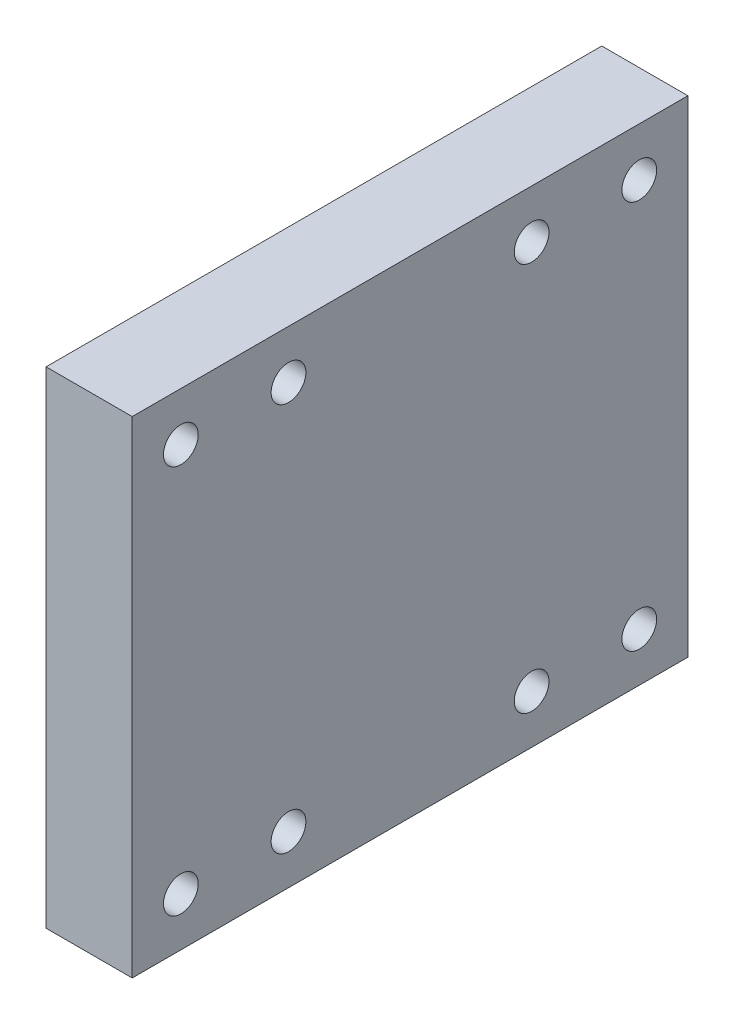
SolidWorks part; units mm, degrees
ref_plane "前视基准面" through (0, 0, 0) normal (0, 0, 1) x (1, 0, 0)
ref_plane "上视基准面" through (0, 0, 0) normal (0, 1, 0) x (1, 0, 0)
ref_plane "右视基准面" through (0, 0, 0) normal (1, 0, 0) x (0, 0, -1)
sketch "草图1" plane through (0, 0, 0) normal (1, 0, 0) x (0, 0, -1)
  line L1 (-40, 35) -> (40, 35)
  line L2 (-40, 35) -> (-40, -35)
  line L3 (-40, -35) -> (40, -35)
  line L4 (40, 35) -> (40, -35)
  line L5 (-40, 35) -> (40, -35) construction
  line L6 (-40, -35) -> (40, 35) construction
  point P0 (0, 0)
  dimension "D1" = 80
  dimension "D2" = 70
extrude "凸台-拉伸1" add sketch "草图1" along normal blind 12.4
hole_wizard "M6 螺纹孔1" positions "草图2" profile "草图3" tap size "M6" standard "GB"
sketch "草图2" plane through (12.4, 0, 0) normal (1, 0, 0) x (0, 0, -1)
  line L0 (0, 40.8734) -> (0, 0) construction
  line L1 (0, 0) -> (49.0326, 0) construction
  point P0 (-17.5, 28)
  point P2 (17.5, 28)
  point P4 (-17.5, -28)
  point P6 (17.5, -28)
  dimension "D1" = 35
  dimension "D2" = 56
sketch "草图3" plane through (12.4, 28, 17.5) normal (0, 1, 0) x (0, 0, -1)
  line L0 (0, 0) -> (0, 16.5022)
  line L1 (0, 16.5022) -> (2.5, 15)
  line L2 (2.5, 15) -> (2.5, 0)
  line L5 (2.5, 0) -> (0, 0)
  line L10 (0, 16.5022) -> (-2.5, 15) construction
  line L11 (0, -6.35) -> (0, 107.95) construction
  dimension "螺纹孔钻头直径" = 5
  dimension "螺纹孔钻头深度" = 15
  dimension "导头角度" = 118
cosmetic thread "孔螺蚊线1" parameters "D1"=10, "D2"=6
cosmetic thread "孔螺蚊线2" parameters "D1"=10, "D2"=6
cosmetic thread "孔螺蚊线3" parameters "D1"=10, "D2"=6
cosmetic thread "孔螺蚊线4" parameters "D1"=10, "D2"=6
hole_wizard "M6 螺纹孔2" positions "草图4" profile "草图5" tap size "M6" standard "GB" end condition through all
sketch "草图4" plane through (12.4, 0, 0) normal (1, 0, 0) x (0, 0, -1)
  line L0 (0, 43.6747) -> (0, 0) construction
  line L1 (0, 0) -> (48.979, 0) construction
  point P0 (-33, 28)
  point P2 (-33, -28)
  point P4 (33, -28)
  point P6 (33, 28)
  dimension "D1" = 66
  dimension "D2" = 56
sketch "草图5" plane through (12.4, 28, 33) normal (0, 1, 0) x (0, 0, -1)
  line L0 (0, 0) -> (0, 12.4)
  line L1 (0, 12.4) -> (2.5, 12.4)
  line L2 (2.5, 12.4) -> (2.5, 0)
  line L5 (2.5, 0) -> (0, 0)
  line L11 (0, -6.35) -> (0, 107.95) construction
  dimension "通孔螺纹孔钻头直径" = 5
  dimension "通孔螺纹孔钻头深度" = 12.4
cosmetic thread "孔螺蚊线5" parameters "D2"=6
cosmetic thread "孔螺蚊线6" parameters "D2"=6
cosmetic thread "孔螺蚊线7" parameters "D2"=6
cosmetic thread "孔螺蚊线8" parameters "D2"=6
